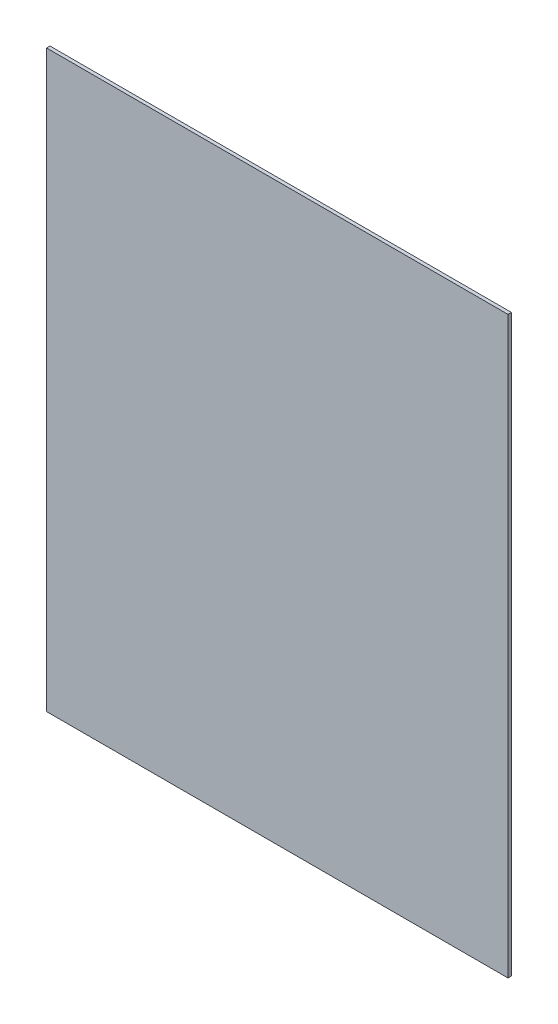
SolidWorks part; units mm, degrees
material "PMMA(有机玻璃)"
ref_plane "前视" through (0, 0, 0) normal (0, 0, 1) x (1, 0, 0)
ref_plane "上视" through (0, 0, 0) normal (0, 1, 0) x (1, 0, 0)
ref_plane "右视" through (0, 0, 0) normal (1, 0, 0) x (0, 0, -1)
sketch "草图1" plane through (0, 0, 0) normal (0, 0, 1) x (1, 0, 0)
  line L1 (-338, 421) -> (338, 421)
  line L2 (-338, 421) -> (-338, -421)
  line L3 (-338, -421) -> (338, -421)
  line L4 (338, 421) -> (338, -421)
  line L5 (-338, 421) -> (338, -421) construction
  line L6 (-338, -421) -> (338, 421) construction
  point P0 (0, 0)
  dimension "D1" = 842
  dimension "D2" = 676
extrude "凸台-拉伸1" add sketch "草图1" along normal blind 5
hole_wizard "M5 间隙孔1" positions "草图3" profile "草图2" hole size "M5" standard "GB"
sketch "草图3" plane through (0, 0, 5) normal (0, 0, 1) x (1, 0, 0)
  line L0 (-427.5, 273) -> (-427.5, -273) construction
  line L1 (-427.5, -273) -> (427.5, -273) construction
  line L2 (0, 273) -> (0, -273) construction
  line L3 (427.5, 273) -> (-427.5, 273) construction
  line L5 (-427.5, 0) -> (427.5, 0) construction
  line L6 (427.5, -273) -> (427.5, 273) construction
  point P0 (-375, -261)
  point P46 (415.5, 250)
  point P48 (-415.5, 250)
  point P58 (-125, -261)
  point P59 (125, -261)
  point P61 (-125, 261)
  point P62 (125, 261)
  point P64 (-375, 261)
  point P88 (375, -261)
  point P89 (375, 261)
  point P108 (415.5, 0)
  point P109 (-415.5, 0)
  point P110 (415.5, -250)
  point P111 (-415.5, -250)
  dimension "D1" = 12
  dimension "D2" = 12
  dimension "D5" = 3
  dimension "D3" = 12
  dimension "D6" = 4
  dimension "D4" = 2
sketch "草图2" plane through (-375, -261, 5) normal (1, 0, 0) x (0, -1, 0)
  line L0 (0, 0) -> (0, 5)
  line L1 (0, 5) -> (2.75, 5)
  line L2 (2.75, 5) -> (2.75, 0)
  line L5 (2.75, 0) -> (0, 0)
  line L11 (0, -6.35) -> (0, 107.95) construction
  dimension "通孔孔直径" = 5.5
  dimension "通孔孔深度" = 5
